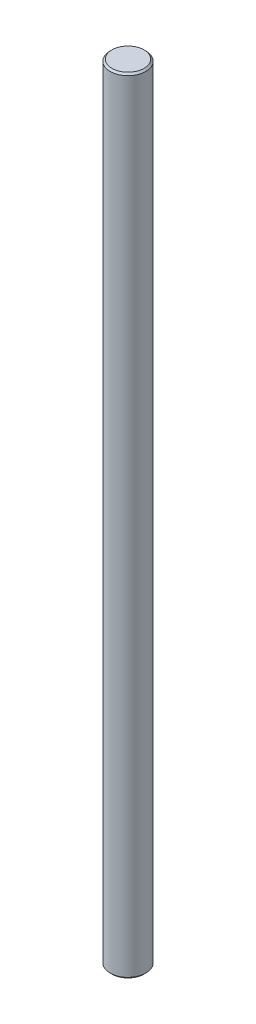
SolidWorks part; units mm, degrees
ref_plane "Front Plane" through (0, 0, 0) normal (0, 0, 1) x (1, 0, 0)
ref_plane "Top Plane" through (0, 0, 0) normal (0, 1, 0) x (1, 0, 0)
ref_plane "Right Plane" through (0, 0, 0) normal (1, 0, 0) x (0, 0, -1)
sketch "Sketch1" plane through (0, 0, 0) normal (0, 1, 0) x (1, 0, 0)
  circle A0 centre (0, 0) radius 5
  dimension "D1" = 10
extrude "Boss-Extrude1" add sketch "Sketch1" along normal blind 220
chamfer "Chamfer1" distance 0.5 angle 45 2 edges at (0, 0, 5) (0, 220, 5)
sketch "Sketch2" plane through (0, 0, 0) normal (0, 1, 0) x (1, 0, 0)
  line L0 (-2.1794, 4.5) -> (2.1794, 4.5)
  circle A0 centre (0, 0) radius 5 construction
  arc A1 (2.1794, 4.5) -> (-2.1794, 4.5) centre (0, 0) ccw
  dimension "D1" = 4.5
extrude "Cut-Extrude1" cut sketch "Sketch2" along normal blind 12
